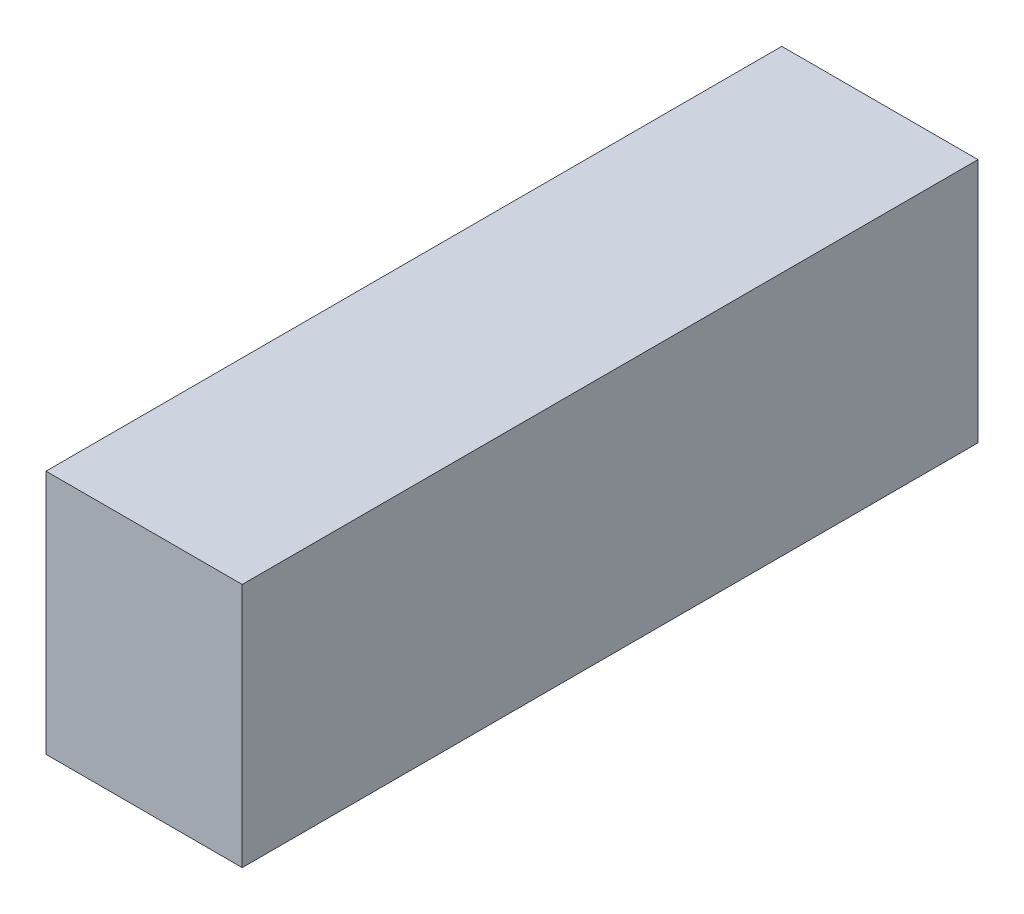
from build123d import *

# Parameters (mm, degrees)
SKETCH1_W           = 8
SKETCH1_H           = 30
BOSS_EXTRUDE1_DEPTH = 10


with BuildPart() as part:
    # Sketch1 → Boss-Extrude1 (new body)
    with BuildSketch(Plane(origin=(0, 0, 0), x_dir=(1, 0, 0), z_dir=(0, 1, 0))):
        Rectangle(SKETCH1_W, SKETCH1_H)
    extrude(amount=BOSS_EXTRUDE1_DEPTH)


solid = part.part
